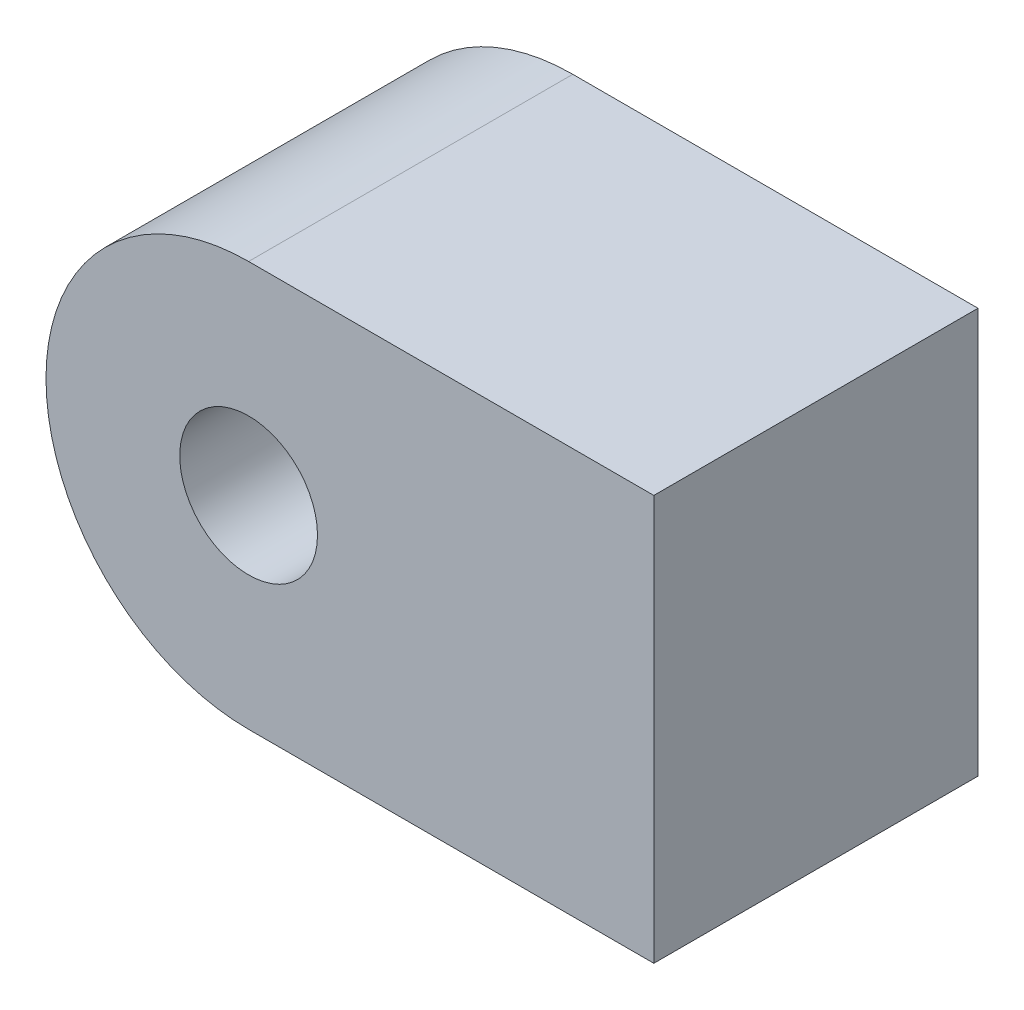
SolidWorks part; units mm, degrees
ref_plane "前视基准面" through (0, 0, 0) normal (0, 0, 1) x (1, 0, 0)
ref_plane "上视基准面" through (0, 0, 0) normal (0, 1, 0) x (1, 0, 0)
ref_plane "右视基准面" through (0, 0, 0) normal (1, 0, 0) x (0, 0, -1)
other "Configuration Table"
sketch "草图1" plane through (0, 0, 0) normal (0, 0, 1) x (1, 0, 0)
  line L0 (0, 15) -> (30, 15)
  line L1 (30, 15) -> (30, -15)
  line L2 (30, -15) -> (0, -15)
  arc A0 (0, -15) -> (0, 15) centre (0, 0) cw
  circle A1 centre (0, 0) radius 5.1
  point P0 (0, 0)
  dimension "D1" = 10.2
  dimension "D2" = 15
  dimension "D3" = 30
extrude "凸台-拉伸1" add sketch "草图1" against normal mid plane 24
